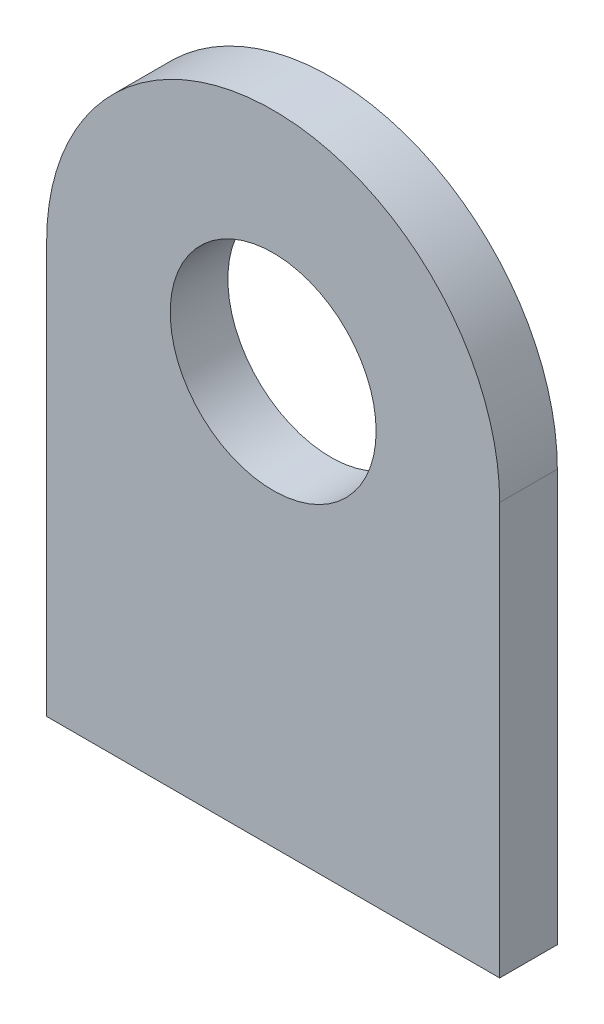
SolidWorks part; units mm, degrees
ref_plane "Front Plane" through (0, 0, 0) normal (0, 0, 1) x (1, 0, 0)
ref_plane "Top Plane" through (0, 0, 0) normal (0, 1, 0) x (1, 0, 0)
ref_plane "Right Plane" through (0, 0, 0) normal (1, 0, 0) x (0, 0, -1)
sketch "Sketch1" plane through (0, 0, 0) normal (0, 0, 1) x (1, 0, 0)
  line L0 (-55, 0) -> (-55, -100)
  line L1 (-55, -100) -> (55, -100)
  line L2 (55, -100) -> (55, 0)
  arc A0 (55, 0) -> (-55, 0) centre (0, 0) ccw
  circle A1 centre (0, 0) radius 25
  dimension "D1" = 50
  dimension "D2" = 110
  dimension "D3" = 100
extrude "Boss-Extrude1" add sketch "Sketch1" along normal blind 14
